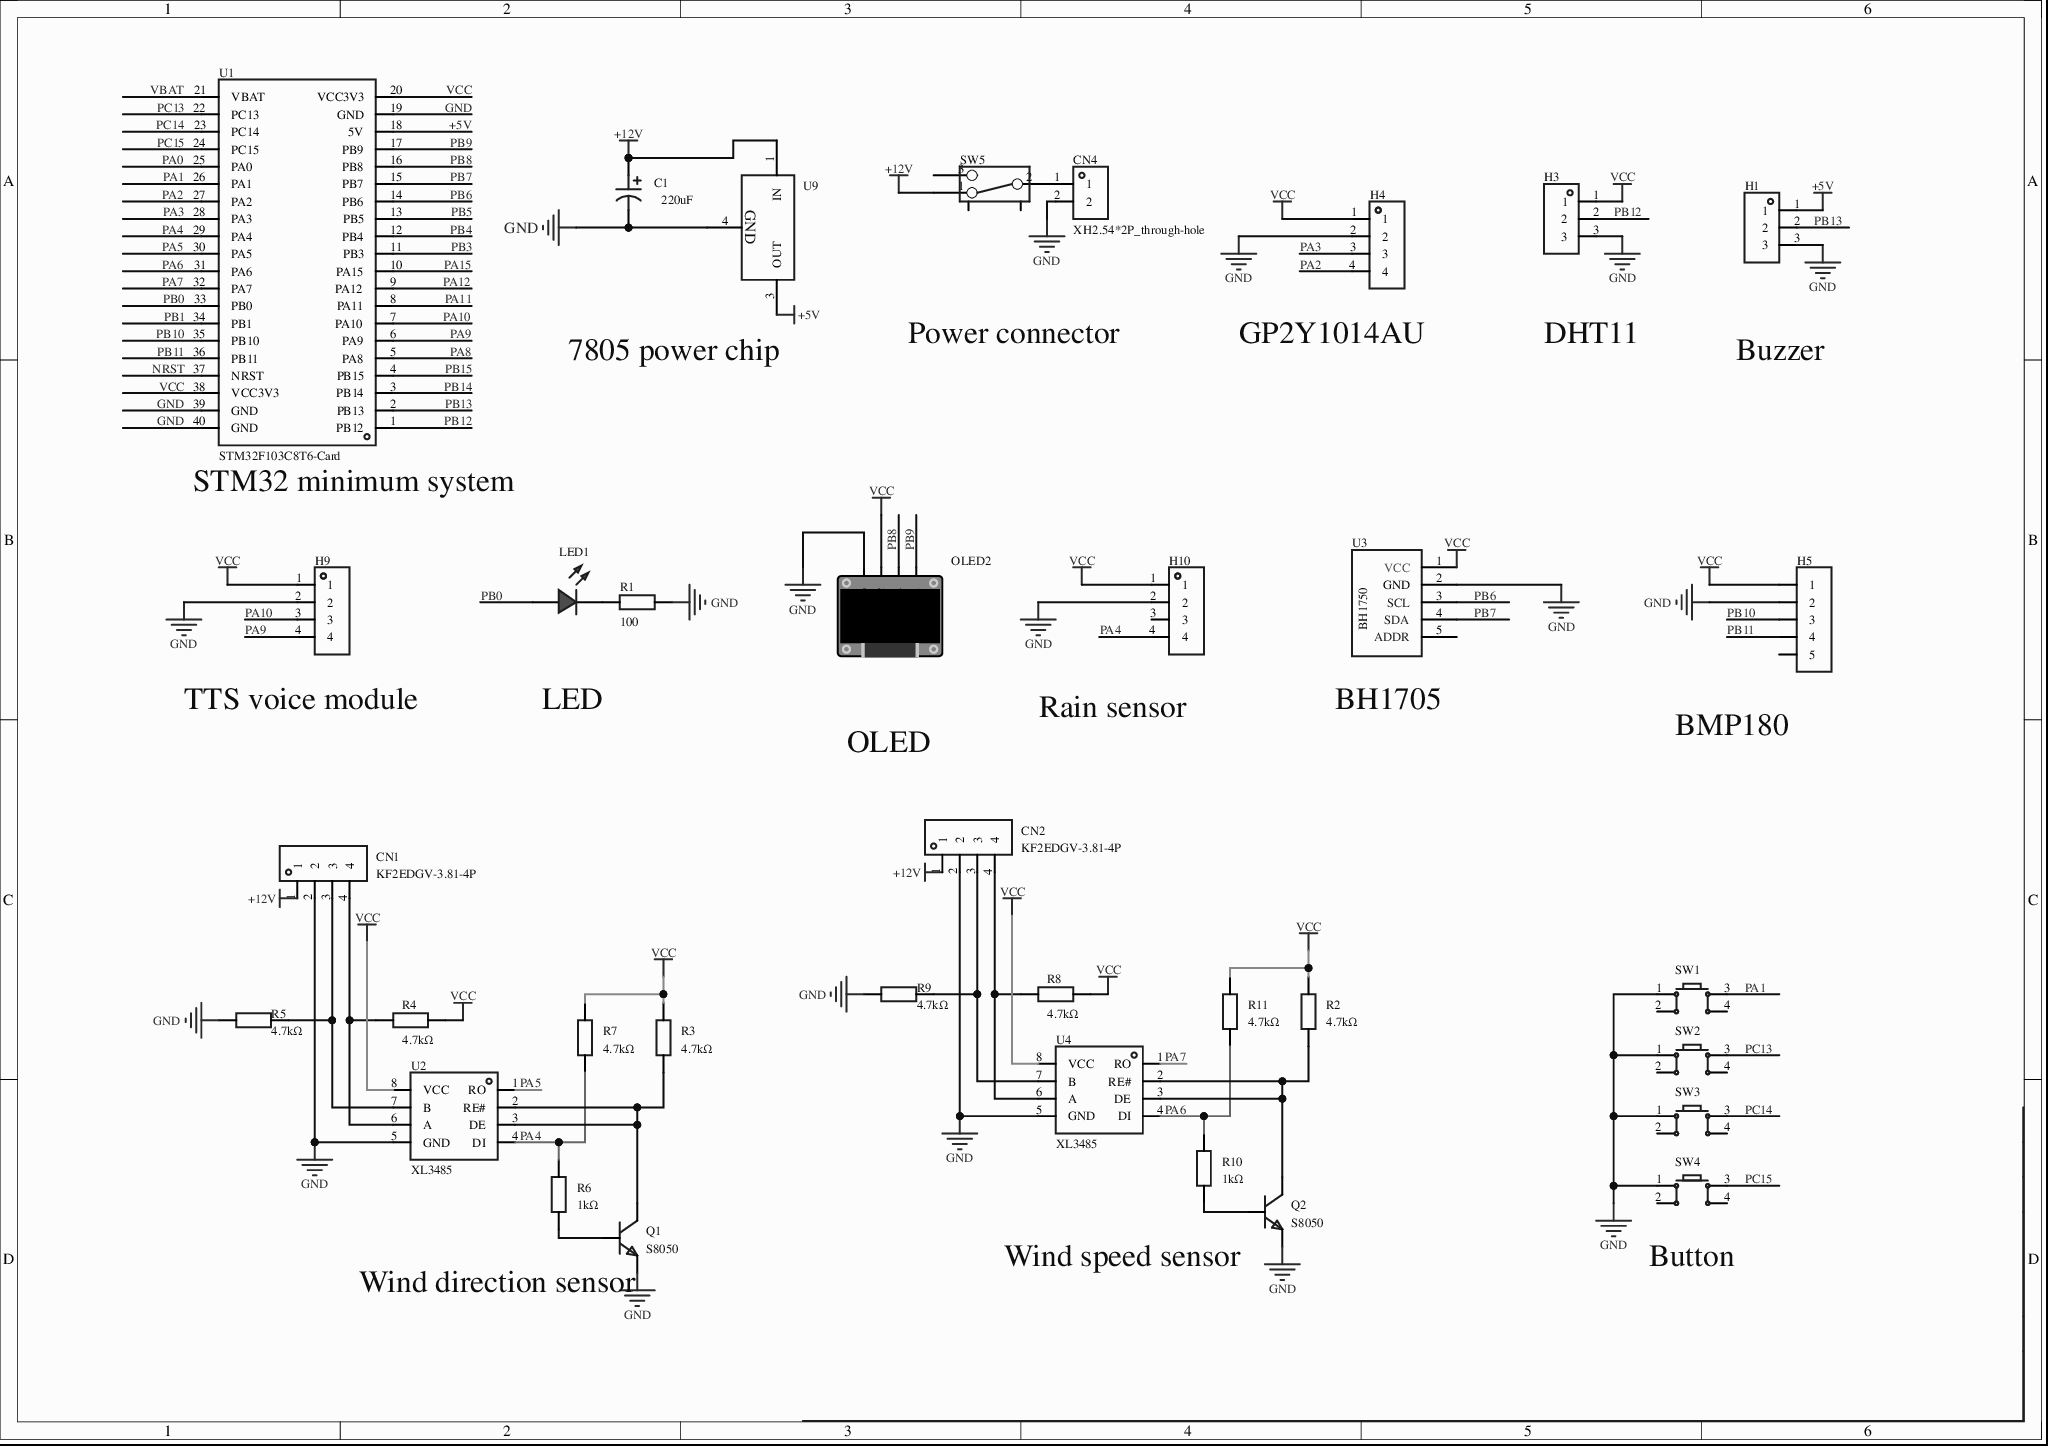
[diagram p0: MISC51967-3.schdoc]
# Altium project MISC51967-2.PrjPcb
1 sheet, 35 parts. Net scope: global (net labels, ports and power ports of the same name join across sheets).
Board file: MISC51967.pcbdoc

## Sheet MISC51967-3.schdoc
size 297 x 209 mm; Version: V1.0; @Project Name: MISC51967; @Page Count: 1; @Update Date: 2026-04-30; @Create Date: 2026-04-30; @Schematic Name: MISC51967; @Page No: 1; @Create Time: 23:22:16; @Update Time: 17:32:40; @Board Name: MISC51967

### Parts
C1  value 220uF  [CAP-SMD_BD8.0-L8.3-W8.3-LS9.3-FD]
CN1  KF2EDGV-3.81-4P  [CONN-TH_4P-P3.81_KF2EDGV-3.81-4P]
CN2  KF2EDGV-3.81-4P  [CONN-TH_4P-P3.81_KF2EDGV-3.81-4P]
CN4  XH2.54*2P_through-hole  [CONN-TH_2P-P2.50-XH2.54-2P]
H1  (no value)  [HDR-TH_3P-P2.54-V-F]
H3  (no value)  [HDR-TH_3P-P2.54-V-F]
H4  (no value)  [HDR-TH_4P-P2.54-V-F]
H5  (no value)  [HDR-TH_5P-P2.54-V-F]
H9  (no value)  [HDR-TH_4P-P2.54-V-F]
H10  (no value)  [HDR-TH_4P-P2.54-V-F]
LED1  (no value)  [LED_TH-3mm]
OLED2  (no value)  [0.96OLED_4P]
Q1  S8050  [SOT-523-3_L1.6-W0.8-P0.50-LS1.6-BR]
Q2  S8050  [SOT-523-3_L1.6-W0.8-P0.50-LS1.6-BR]
R1  100  [Res_1/8W]
R2  4.7kΩ  [R0402ST]
R3  4.7kΩ  [R0402ST]
R4  4.7kΩ  [R0402ST]
R5  4.7kΩ  [R0402ST]
R6  1kΩ  [R0402ST]
R7  4.7kΩ  [R0402ST]
R8  4.7kΩ  [R0402ST]
R9  4.7kΩ  [R0402ST]
R10  1kΩ  [R0402ST]
R11  4.7kΩ  [R0402ST]
SW1  (no value)  [SW-TH_4P-L6.0-W6.0-P4.50-LS6.5]
SW2  (no value)  [SW-TH_4P-L6.0-W6.0-P4.50-LS6.5]
SW3  (no value)  [SW-TH_4P-L6.0-W6.0-P4.50-LS6.5]
SW4  (no value)  [SW-TH_4P-L6.0-W6.0-P4.50-LS6.5]
SW5  (no value)  [拨动开关]
U1  STM32F103C8T6-Card  [CONN-TH_L53.3-W22.9_STM32F103C8T6-CARD]
U2  XL3485  [SOP-8_L5.0-W4.0-P1.27-LS6.0-BL]
U3  (no value)  [BH1750光照传感器]
U4  XL3485  [SOP-8_L5.0-W4.0-P1.27-LS6.0-BL]
U9  L78M05ABDT-TR  [TO-252-2_L6.5-W6.1-P4.58-LS10.0-TL]  (value not drawn)

### Nets
+5V: H1.1 U1.18(5V) U9.3(OUT)
+12V: C1.1 CN1.1 CN2.1 SW5.1 U9.1(IN)
GND: C1.2 CN1.2 CN2.2 CN4.2 H1.3 H3.3 H4.2 H5.2 H9.2 H10.2 OLED2.1(GND) Q1.2(E) Q2.2(E) R1.2 R5.1 R9.1 SW1.1 SW2.1 SW3.1 SW4.1 U1.19(GND) U1.39(GND) U1.40(GND) U2.5(GND) U3.2(GND) U4.5(GND) U9.4(GND)
VCC: H3.1 H4.1 H5.1 H9.1 H10.1 OLED2.2(VCC) R2.1 R3.1 R4.2 R7.1 R8.2 R11.1 U1.20(VCC3V3) U1.38(VCC3V3) U2.8(VCC) U3.1(VCC) U4.8(VCC)
NRST: U1.37(NRST)
PA0: U1.25(PA0)
PA1: SW1.3 U1.26(PA1)
PA2: H4.4 U1.27(PA2)
PA3: H4.3 U1.28(PA3)
PA4: H10.4 R6.2 R7.2 U1.29(PA4) U2.4(DI)
PA5: U1.30(PA5) U2.1(RO)
PA6: R10.2 R11.2 U1.31(PA6) U4.4(DI)
PA7: U1.32(PA7) U4.1(RO)
PA8: U1.5(PA8)
PA9: H9.4 U1.6(PA9)
PA10: H9.3 U1.7(PA10)
PA11: U1.8(PA11)
PA12: U1.9(PA12)
PA15: U1.10(PA15)
PB0: LED1.1(C) U1.33(PB0)
PB1: U1.34(PB1)
PB3: U1.11(PB3)
PB4: U1.12(PB4)
PB5: U1.13(PB5)
PB6: U1.14(PB6) U3.3(SCL)
PB7: U1.15(PB7) U3.4(SDA)
PB8: OLED2.3(SCL) U1.16(PB8)
PB9: OLED2.4(SDA) U1.17(PB9)
PB10: H5.3 U1.35(PB10)
PB11: H5.4 U1.36(PB11)
PB12: H3.2 U1.1(PB12)
PB13: H1.2 U1.2(PB13)
PB14: U1.3(PB14)
PB15: U1.4(PB15)
PC13: SW2.3 U1.22(PC13)
PC14: SW3.3 U1.23(PC14)
PC15: SW4.3 U1.24(PC15)
VBAT: U1.21(VBAT)
NetCN1_3: CN1.3 R5.2 U2.7(B)
NetCN1_4: CN1.4 R4.1 U2.6(A)
NetCN2_3: CN2.3 R9.2 U4.7(B)
NetCN2_4: CN2.4 R8.1 U4.6(A)
NetCN4_1: CN4.1 SW5.2
NetLED1_2: LED1.2(A) R1.1
NetQ1_1: Q1.1(B) R6.1
NetQ1_3: Q1.3(C) R3.2 U2.2(RE#) U2.3(DE)
NetQ2_1: Q2.1(B) R10.1
NetQ2_3: Q2.3(C) R2.2 U4.2(RE#) U4.3(DE)

Not connected (* = marked no-connect by the designer): H5 5; H10 3; SW1 2 4; SW2 2 4; SW3 2 4; SW4 2 4; SW5 3 4 5; U3 5(ADDR)

### Notes on the sheet
- STM32最小系统板
  豆包出来的
  串口：
  PM2.5
  TTS语音模块
  GPIO:
  LED灯：一个
  按键开关：四个
  IIC:
  0.96英寸OLED显示屏
  BMP180气压模块
  BH1750光照传感器
  One-Wire:
  DHT11
  雨水传感器
  蜂鸣器
  LED
  按键
  2路RS485:
  风速传感器
  风向传感器
- Power connector
- (near H4) GP2Y1014AU
- DHT11
- (near U9) 7805 power chip
- Buzzer
- (near U1) STM32 minimum system
- (near H9) TTS voice module
- LED
- OLED
- (near H10) Rain sensor
- (near U3) BH1705
- (near H5) BMP180
- (near Q1) Wind direction sensor
- (near Q2) Wind speed sensor
- (near SW4) Button

### Library data of the parts
C1 = EMK1VM221FB0D00R: 容值:220uF;精度:±20%;额定电压:35V;电容体直径:-;电容体长度:-;纹波电流:-;等效串联电阻:-;工作寿命:-;工作温度:-;; Manufacturer: AISHI(艾华集团); 3D Model: ae37c166a99f49b1b935231edf05d58d; 3D Model Transform: 366.1,326.8,0,0,0,0,0,0,0; Tolerance: ±20%; Rated Voltage: 35V; AddInBom: yes; Symbol: EMK1VM221FB0D00R; Device: EMK1VM221FB0D00R; LCSC Part Name: 220uF ±20% 35V; Supplier Part: C724731; Manufacturer Part: EMK1VM221FB0D00R; Supplier Footprint: SMD,8x10.5mm; JLCPCB Part Class: Extended Part; Datasheet: https://atta.szlcsc.com/upload/public/pdf/source/20200818/C724731_E3C3C738DF50876976EE53B5D20E1717.pdf; Supplier: LCSC; φD: -; L: -; Ripple Current: -; Equivalent Series Resistance(ESR): -; Lifetime @ Temp: -; Operating Temperature: -; ConvertToPcb: yes; FootprintName: CAP-SMD_BD8.0-L8.3-W8.3-LS9.3-FD; ModelName: CAP-SMD_BD8.0-L8.3-W8.3-LS9.3-FD
CN1 CN2 = KF2EDGV-3.81-4P: Symbol: KF2EDGV-3.81-4P_C9900017457; AddInBom: yes; ModelId: c22b1d4a74cc44ef9907503feccb8f480819f05c4eef4c71ace90d822a990e87; ModelTransform: 631.4948,283.50337,0,0,0,0,0,-23.622,-137.795; Device: KF2EDGV-3.81-4P; LCSC Part Name: KF2EDGV-3.81-4P; SupplierPart: C9900017457; ManufacturerPart: KF2EDGV-3.81-4P; Supplier Footprint: CONN-TH_4P-P3.81_KF2EDGV-3.81-4P; JLCPCB Part Class: Extended Part; Supplier: LCSC; ConvertToPcb: yes; FootprintName: CONN-TH_4P-P3.81_KF2EDGV-3.81-4P; ModelName: CONN-TH_4P-P3.81_KF2EDGV-3.81-4P
CN4 = XH2.54*2P_直插: 3D Model: 325c595e30db4df8abe76612dd40b0fa0819f05c4eef4c71ace90d822a990e87; 3D Model Transform: 295.275,228.346,0,180,0,0,-0.002,-20.079,-137.795; AddInBom: yes; Device: XH2.54*2P_through-hole; Symbol: XH2.54*2P_through-hole; LCSC Part Name: XH2.54*2P_直插; Supplier Part: C9900008615; Manufacturer Part: XH2.54*2P_直插; Supplier Footprint: XH2.54_2P; JLCPCB Part Class: Extended Part; Supplier: LCSC; FootprintName: CONN-TH_2P-P2.50-XH2.54-2P; ConvertToPcb: yes; ModelName: CONN-TH_2P-P2.50-XH2.54-2P
H1 H3 = HDR-F_2.54_1x3P: Symbol: PM254V-11-03-H85; 3D Model: f3b3cc5aae9641bf9e56fc160cef875b; 3D Model Transform: 299.9994,100,0,0,0,0,0,0,-118.11; ConvertToPcb: yes; ModelName: HDR2.54-F-LI-1X3P; Device: HDR-F_2.54_1x3P; Supplier Part: C541850; Supplier Footprint: 插件; FootprintName: HDR-TH_3P-P2.54-V-F; AddInBom: yes
H4 = HDR-F_2.54_1x4P: Symbol: 2.54-1*4P female; ConvertToPcb: yes; ModelId: d187812051054f85879fcaa51a310d8e0819f05c4eef4c71ace90d822a990e87; ModelTransform: 419.6842,98.464,0,0,0,0,0,0,-118.11; Device: HDR-F_2.54_1x4P; FootprintName: HDR-TH_4P-P2.54-V-F; AddInBom: yes; SupplierPart: C2718488; Supplier Footprint: 插件; ModelName: HDR-TH_4P-P2.54-V-F
H5 = HDR-F_2.54_1x5P: Symbol: Header-Female-2.54_1x5; ConvertToPcb: yes; ModelId: f49cb6116a3d45e5a64915bf3e00773f; ModelTransform: 519.684,98.464,0,0,0,0,0,0,-124.016; Device: HDR-F_2.54_1x5P; AddInBom: yes; SupplierPart: C50950; Supplier Footprint: 插件; FootprintName: HDR-TH_5P-P2.54-V-F; ModelName: HDR-TH_5P-P2.54-V-F
H9 H10 = HDR-F_2.54_1x4P: Symbol: 2.54-1*4P female; 3D Model: d187812051054f85879fcaa51a310d8e0819f05c4eef4c71ace90d822a990e87; 3D Model Transform: 419.6842,98.464,0,0,0,0,0,0,-118.11; ConvertToPcb: yes; Device: HDR-F_2.54_1x4P; Supplier Part: C2718488; Supplier Footprint: 插件; FootprintName: HDR-TH_4P-P2.54-V-F; AddInBom: yes; ModelName: HDR-TH_4P-P2.54-V-F
LED1 = LED_TH-R_3mm: ConvertToPcb: yes; ModelId: a497c992633541038a38947cdc58012f0819f05c4eef4c71ace90d822a990e87; ModelName: LED-TH-3mm_R; ModelTransform: 141.274,153.327,0,0,0,0,-5.984,0,-137.795; Symbol: LED_TH-R; Device: LED_TH-R_3mm; AddInBom: yes; FootprintName: LED_TH-3mm; Supplier Footprint: 插件
OLED2 = 0.96OLED模块_4P: 3D Model: 79c000fdb68d45a296c2e9bedf4f9055; 3D Model Transform: 1393.69792,1318.895,0,0,0,0,0,-560.079,-137.795; ConvertToPcb: yes; Symbol: 0.96OLED模块_4P; Device: 0.96OLED模块_4P; Supplier Footprint: 插件; AddInBom: yes; FootprintName: 0.96OLED_4P; ModelName: 0.96OLED_4P
Q1 Q2 = S8050_C19630847: Manufacturer: YONGYUTAI(永裕泰); 3D Model: 52d9edd53d874f49a5800237040977fe; 3D Model Transform: 57.0865,66.929,0,0,0,0,0,0,0; AddInBom: yes; Symbol: S8050_C19630847; Device: S8050_C19630847; LCSC Part Name: S8050; Supplier Footprint: SOT-523; Datasheet: https://atta.szlcsc.com/upload/public/pdf/source/20231208/234EFAE5DDDACC028C97F827503C8536.pdf; Supplier: LCSC; Supplier Part: C19630847; Manufacturer Part: S8050; ConvertToPcb: yes; FootprintName: SOT-523-3_L1.6-W0.8-P0.50-LS1.6-BR; ModelName: SOT-523-3_L1.6-W0.8-P0.50-LS1.6-BR
R1 = Res_AXIAL-1/8W: Symbol: Resistor; ConvertToPcb: yes; ModelId: b2b5ae7ae4c642178fe0039925c86a3f0819f05c4eef4c71ace90d822a990e87; ModelName: RES-TH_BD1.8-L3.2-P7.20-D0.4; ModelTransform: 282.86,66.88,253.09,0,0,0,0,0,-191; Device: Res_AXIAL-1/8W; Value: 100; AddInBom: yes; Supplier Footprint: 轴向引线; FootprintName: Res_1/8W
R2-R11 = R0402S (私有库): Manufacturer: Kind Elecs.; Symbol: R0402S (private library); 3D Model: 671aefced39d4c318694bba8bd8efd39; 3D Model Transform: 39.37,19.685,0,0,0,0,0,0.0005,0; AddInBom: yes; ModelName: R0402_L1.0-W0.5-H0.5; Device: R0402S (private library); Supplier Footprint: 0402; JLCPCB Part Class: Private library; Datasheet: https://atta.szlcsc.com/upload/public/pdf/source/20170606/1496716515432.pdf; Type: Thick film resistor; ConvertToPcb: yes; FootprintName: R0402ST
  R2-R5 R7-R9 R11: Value: 4.7kΩ
  R6 R10: Value: 1kΩ
SW1-SW4 = Key_TH_6x6x6: 触点电流:50mA;额定电压(DC):12V;绝缘电阻:100MΩ;电路结构:单刀单掷;安装方式:直插;按钮形状:圆形按钮;按钮/盖帽颜色:黑色;作用力:260gf@±30gf;工作温度:-25℃~+70℃;引脚样式:PC引脚;开关长度:6mm;开关宽度:6mm;开关高度:6mm;带支架:否;; Symbol: Tactile switch; 3D Model: 20eee248bc684ccd8cbdbb1d0d91ec6f0819f05c4eef4c71ace90d822a990e87; 3D Model Transform: 236.22,323.03,0,90,0,0,0,0,-137.795; AddInBom: yes; ModelName: SW-TH_4P-L6.0-W6.0-H5.0-LS6.5-P4.50; Device: Key_TH_6x6x6; Supplier Footprint: 插件; FootprintName: SW-TH_4P-L6.0-W6.0-P4.50-LS6.5; ConvertToPcb: yes
SW5 = 拨动开关_正: Device: Toggle switch_positive; Symbol: Toggle switch; ConvertToPcb: yes; ModelId: 4321fe59a4074cbfb4989553f297c68f0819f05c4eef4c71ace90d822a990e87; ModelName: SW-TH_SS-12D02-VG4; ModelTransform: 370.09,208.7,472.35,0,0,0,0,0,-110; FootprintName: Toggle switch; AddInBom: yes; Supplier Footprint: 插件
U1 = STM32F103C8T6-Card: AddInBom: yes; Device: STM32F103C8T6-Card; Symbol: STM32F103C8T6-CARD; FootprintName: CONN-TH_L53.3-W22.9_STM32F103C8T6-CARD; LCSC Part Name: STM32F103C8T6-Card; SupplierPart: C9900077949; ManufacturerPart: STM32F103C8T6-Card; Supplier Footprint: 插件; Supplier: LCSC; ConvertToPcb: yes
U2 U4 = XL3485: 收发器 驱动器/接收器：1/1 数据速率：10Mbps 电源电压：3V~3.6V; Manufacturer: XINLUDA(信路达); 3D Model: a3315c1c78f949e6bb82c6eaca1c53c7; 3D Model Transform: 244.094,196.85,0,90,0,0,0,0,0; AddInBom: yes; ModelName: SOP-8_L5.0-W4.0-H1.8-LS6.2-P1.27; Symbol: XL3485; Device: XL3485; LCSC Part Name: XD/XL3485 3.3V供电，半双工RS485收发器; Supplier Part: C609753; Manufacturer Part: XL3485; Supplier Footprint: SOP-8; JLCPCB Part Class: Extended library; Datasheet: https://atta.szlcsc.com/upload/public/pdf/source/20230807/BB5221D628ED74149445ABEF162A8932.pdf; Supplier: LCSC; ConvertToPcb: yes; FootprintName: SOP-8_L5.0-W4.0-P1.27-LS6.0-BL
U3 = BH1750光照传感器: Symbol: BH1750 light sensor; AddInBom: yes; Device: BH1750 light sensor; ConvertToPcb: yes; FootprintName: BH1750 light sensor
U9 = L78M05ABDT-TR: L78M Series 500 mA 5 V Three Terminal Positive Voltage LDO Regulator - TO-252; Manufacturer: ST(意法半导体); 3D Model: 6b2ea0154a284e6db98f69bccdba3606; 3D Model Transform: 255.905,390.52442,0,270,0,0,38.183,0.432,0; AddInBom: yes; ModelName: TO-252-2_L6.5-W6.1-H2.3-LS10.0-P4.58; Symbol: L78M05ABDT-TR; Device: L78M05ABDT-TR; LCSC Part Name: L78M05ABDT-TR; Supplier Part: C58069; Manufacturer Part: L78M05ABDT-TR; Supplier Footprint: TO-252-2(DPAK); JLCPCB Part Class: Basic Part; Datasheet: https://atta.szlcsc.com/upload/public/pdf/source/20150912/1457707362652.pdf; Supplier: LCSC; ConvertToPcb: yes; FootprintName: TO-252-2_L6.5-W6.1-P4.58-LS10.0-TL